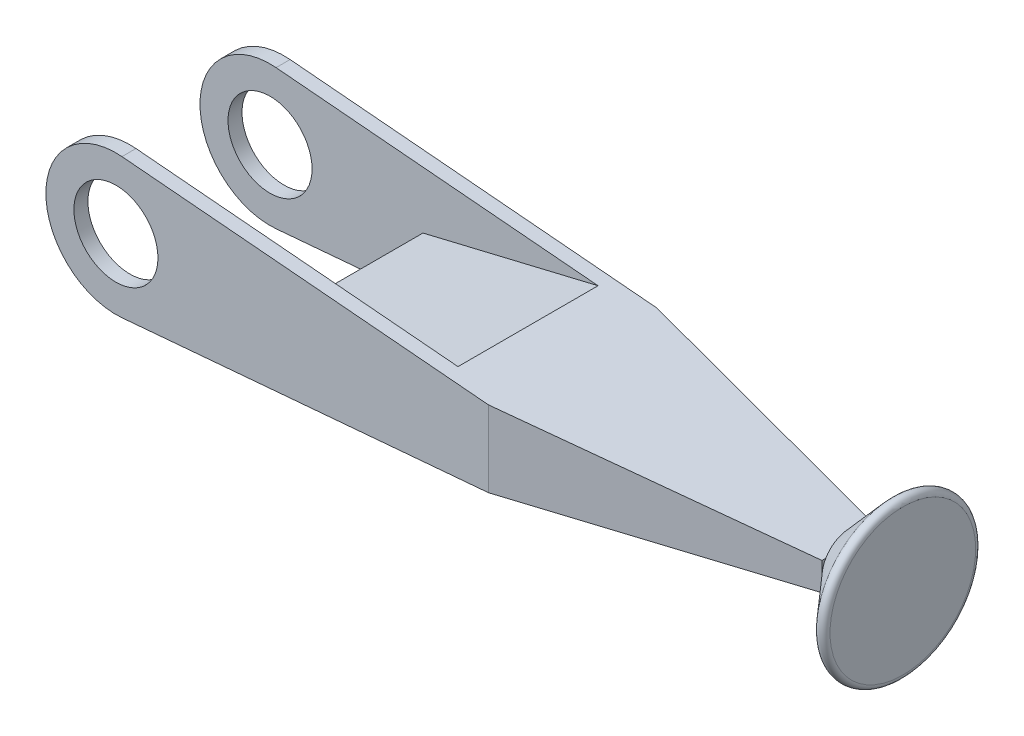
from build123d import *

# Parameters (mm, degrees)
SKETCH13_R          = 15
BOSS_EXTRUDE6_DEPTH = 5
BOSS_EXTRUDE7_DEPTH = 50
BOSS_EXTRUDE8_START = 50
SKETCH15_R          = 15
BOSS_EXTRUDE8_DEPTH = 5
CUT_EXTRUDE2_DEPTH  = 41.5
FILLET2_R           = 2


with BuildPart() as part:
    # Sketch13 → Boss-Extrude6 (new body)
    with BuildSketch(Plane.XY):
        with BuildLine():
            Line((2.157181952, 24.906757437), (232, 5))
            Line((232, 5), (232, -5))
            Line((232, -5), (2.157181952, -24.906757437))
            ThreePointArc((2.157181952, -24.906757437), (-25, 0), (2.157181952, 24.906757437))
        make_face()
        Circle(SKETCH13_R, mode=Mode.SUBTRACT)
    extrude(amount=BOSS_EXTRUDE6_DEPTH)

    # Sketch14 → Boss-Extrude7 (add)
    with BuildSketch(Plane.XY.offset(5)):
        Polygon((232, 5), (117.078590976, 14.953378719), (54.588884616, 0), (117.078590976, -14.953378719), (232, -5), align=None)
    extrude(amount=BOSS_EXTRUDE7_DEPTH)

    # Sketch15 → Boss-Extrude8 (add)
    with BuildSketch(Plane.XY.offset(5).offset(BOSS_EXTRUDE8_START)):
        with BuildLine():
            Line((117.078590976, 14.953378719), (2.157181952, 24.906757437))
            ThreePointArc((2.157181952, 24.906757437), (-25, 0), (2.157181952, -24.906757437))
            Line((2.157181952, -24.906757437), (117.078590976, -14.953378719))
            Line((117.078590976, -14.953378719), (232, -5))
            Line((232, -5), (232, 5))
            Line((232, 5), (117.078590976, 14.953378719))
        make_face()
        Circle(SKETCH15_R, mode=Mode.SUBTRACT)
    extrude(amount=BOSS_EXTRUDE8_DEPTH)

    # Sketch16 → Cut-Extrude2 (cut, symmetric)
    with BuildSketch(Plane(origin=(0, 0, 0), x_dir=(1, 0, 0), z_dir=(0, 1, 0))):
        Polygon((232, 0), (133.011770042, 0), (232, -20), align=None)
        Polygon((232, -40), (232, -60), (133.011770042, -60), align=None)
    extrude(amount=CUT_EXTRUDE2_DEPTH, both=True, mode=Mode.SUBTRACT)

    # Sketch20 → Revolve4 (revolve)
    with BuildSketch(Plane(origin=(0, 0, 0), x_dir=(1, 0, 0), z_dir=(0, 1, 0))):
        Polygon((232, -30), (232, -20), (250.852474196, 1.265966163), (250.852474196, -30), align=None)
    revolve(axis=Axis((250.852474196, 0, 30), (-1, 0, 0)))

    # Fillet2
    fillet2_edges = [part.edges().sort_by_distance(p)[0] for p in [
        (250.852474196, 0, 61.265966163),
    ]]
    fillet(fillet2_edges, radius=FILLET2_R)


solid = part.part
